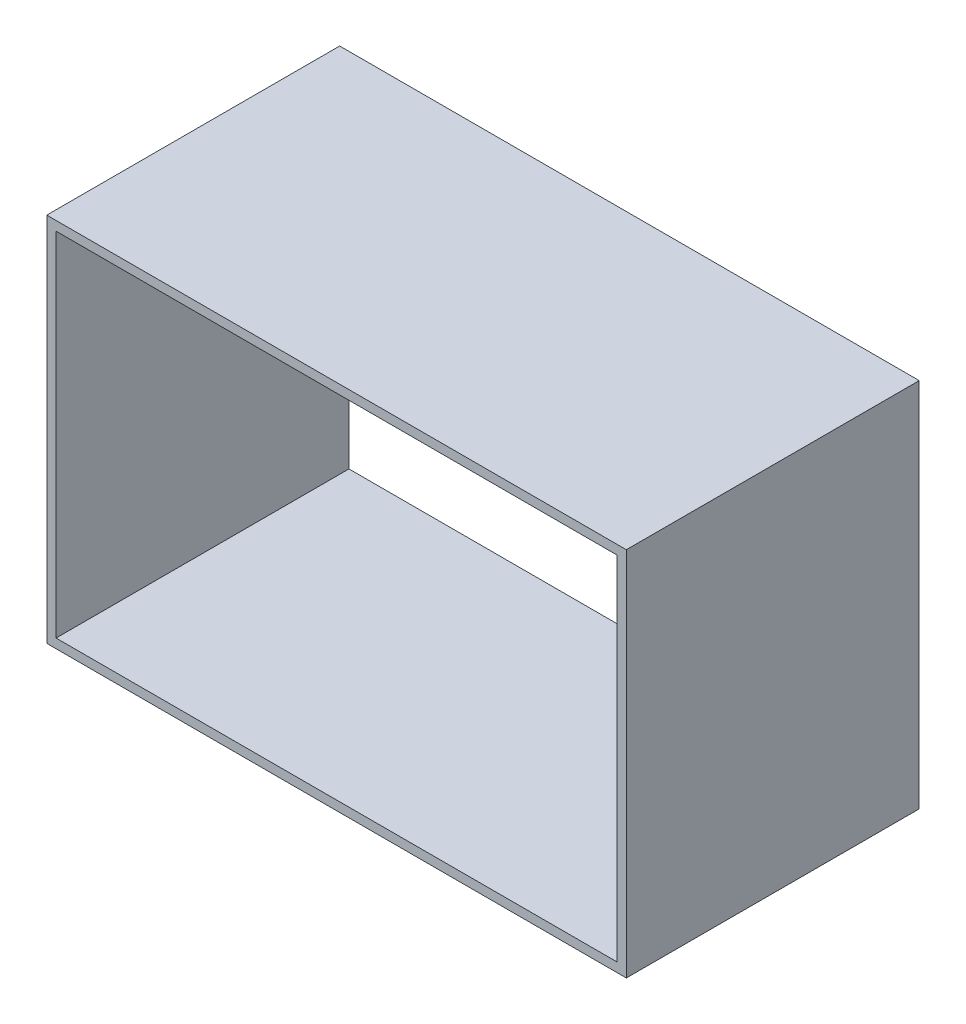
from build123d import *

# Parameters (mm, degrees)
SKETCH1_W           = 500
SKETCH1_H           = 320
SKETCH1_W_2         = 484
SKETCH1_H_2         = 304
BOSS_EXTRUDE1_DEPTH = 252.7


with BuildPart() as part:
    # Sketch1 → Boss-Extrude1 (new body)
    with BuildSketch(Plane.XY):
        with Locations((250, 160)):
            Rectangle(SKETCH1_W, SKETCH1_H)
        with Locations((250, 160)):
            Rectangle(SKETCH1_W_2, SKETCH1_H_2, mode=Mode.SUBTRACT)
    extrude(amount=BOSS_EXTRUDE1_DEPTH)


solid = part.part
